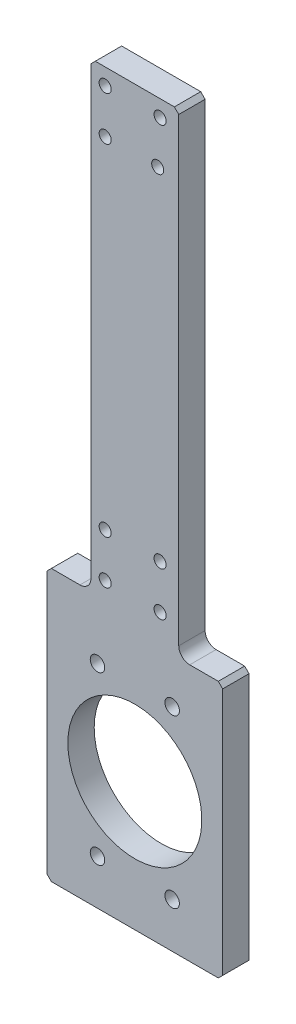
from build123d import *

# Parameters (mm, degrees)
SKETCH_1_W                   = 80
SKETCH_1_H                   = 333.5
EXTRUDE_1_DEPTH              = 12
CHAMFER_1_SIZE               = 2
HOLE_WIZARD_M5_1_D           = 5.5
HOLE_WIZARD_M5_1_CBORE_D     = 10
HOLE_WIZARD_M5_1_CBORE_DEPTH = 5.7
SKETCH_10_W                  = 20
SKETCH_10_H                  = 210
SKETCH_10_H_2                = 216.5
CUT_EXTRUDE_1_DEPTH          = 172.899861838
CHAMFER_2_SIZE               = 2
FILLET_1_R                   = 5
HOLE_WIZARD_M6_1_D           = 6.6
HOLE_WIZARD_M6_1_CBORE_D     = 11
HOLE_WIZARD_M6_1_CBORE_DEPTH = 6.8
SKETCH_14_R                  = 30.5
CUT_EXTRUDE_2_DEPTH          = 172.899861838


with BuildPart() as part:
    # 草图1 → 凸台-拉伸1 (new body)
    with BuildSketch(Plane.XY):
        Rectangle(SKETCH_1_W, SKETCH_1_H)
    extrude(amount=EXTRUDE_1_DEPTH)

    # 倒角1
    chamfer_1_edges = [part.edges().sort_by_distance(p)[0] for p in [
        (-40, -166.75, 6),
        (40, -166.75, 6),
        (40, 166.75, 6),
        (-40, 166.75, 6),
    ]]
    chamfer(chamfer_1_edges, length=CHAMFER_1_SIZE)

    # M5 六角圆柱头螺钉的柱形沉头孔1 (through all)
    with Locations(Plane(origin=(0, 0, 0), x_dir=(-1, 0, 0), z_dir=(0, 0, -1))):
        with Locations((13.5, -35.75), (13.5, 139.25), (-11.5, 159.25), (-10.418856804, 139.25), (13.5, 159.25), (-11.5, -15.75), (13.5, -15.75), (-11.5, -35.75)):
            CounterBoreHole(HOLE_WIZARD_M5_1_D / 2, HOLE_WIZARD_M5_1_CBORE_D / 2, HOLE_WIZARD_M5_1_CBORE_DEPTH)

    # 草图10 → 切除-拉伸1 (cut, through all)
    with BuildSketch(Plane.XY.offset(12)):
        with Locations((-30, 61.75)):
            Rectangle(SKETCH_10_W, SKETCH_10_H)
        with Locations((30, 58.5)):
            Rectangle(SKETCH_10_W, SKETCH_10_H_2)
    extrude(amount=-CUT_EXTRUDE_1_DEPTH, mode=Mode.SUBTRACT)

    # 倒角2
    chamfer_2_edges = [part.edges().sort_by_distance(p)[0] for p in [
        (-40, -43.25, 6),
        (-20, 166.75, 6),
        (40, -49.75, 6),
        (20, 166.75, 6),
    ]]
    chamfer(chamfer_2_edges, length=CHAMFER_2_SIZE)

    # 圆角1
    fillet_1_edges = [part.edges().sort_by_distance(p)[0] for p in [
        (-20, -43.25, 6),
        (20, -49.75, 6),
    ]]
    fillet(fillet_1_edges, radius=FILLET_1_R)

    # M6 六角圆柱头螺钉的柱形沉头孔1 (through all)
    with Locations(Plane(origin=(0, 0, 0), x_dir=(-1, 0, 0), z_dir=(0, 0, -1))):
        with Locations((-17, -70.25), (-17, -146.25), (17, -146.25), (17, -70.25)):
            CounterBoreHole(HOLE_WIZARD_M6_1_D / 2, HOLE_WIZARD_M6_1_CBORE_D / 2, HOLE_WIZARD_M6_1_CBORE_DEPTH)

    # 草图14 → 切除-拉伸2 (cut, through all)
    with BuildSketch(Plane(origin=(0, 0, 0), x_dir=(-1, 0, 0), z_dir=(0, 0, -1))):
        with Locations((0, -108.25)):
            Circle(SKETCH_14_R)
    extrude(amount=-CUT_EXTRUDE_2_DEPTH, mode=Mode.SUBTRACT)


solid = part.part
